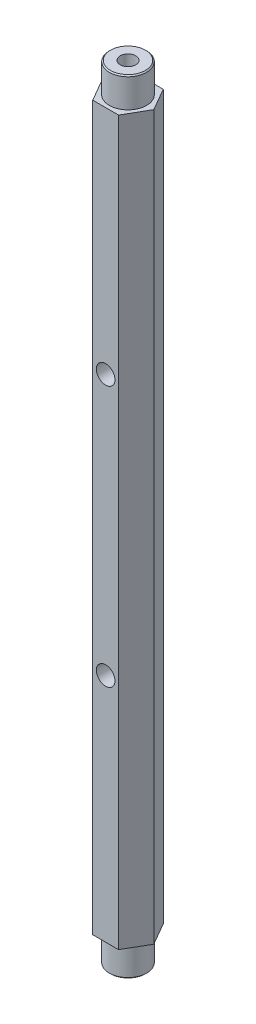
from build123d import *

# Parameters (mm, degrees)
BOSS_EXTRUDE1_DEPTH   = 210
SKETCH2_OUTSIDE_W     = 58.016
SKETCH2_OUTSIDE_H     = 56.16
SKETCH2_OUTSIDE_R     = 5
CUT_EXTRUDE1_DEPTH    = 8
SKETCH3_OUTSIDE_W     = 58.016
SKETCH3_OUTSIDE_H     = 56.16
SKETCH3_OUTSIDE_R     = 5
CUT_EXTRUDE2_DEPTH    = 8
M6_TAPPED_HOLE1_D     = 5
M5_TAPPED_HOLE1_D     = 4.2
M5_TAPPED_HOLE1_DEPTH = 12.4
M5_TAPPED_HOLE1_TIP   = 1.2618073
M5_TAPPED_HOLE2_D     = 4.2
M5_TAPPED_HOLE2_DEPTH = 12.4
M5_TAPPED_HOLE2_TIP   = 1.2618073
CHAMFER1_SIZE         = 0.3


with BuildPart() as part:
    # Sketch1 → Boss-Extrude1 (new body)
    with BuildSketch(Plane(origin=(0, 0, 0), x_dir=(1, 0, 0), z_dir=(0, 1, 0))):
        Polygon((6.92820323, 0), (3.464101615, 6), (-3.464101615, 6), (-6.92820323, 0), (-3.464101615, -6), (3.464101615, -6), align=None)
    extrude(amount=BOSS_EXTRUDE1_DEPTH)

    # Sketch2 outside → Cut-Extrude1 (cut)
    with BuildSketch(Plane(origin=(0, 210, 0), x_dir=(1, 0, 0), z_dir=(0, 1, 0))):
        Rectangle(SKETCH2_OUTSIDE_W, SKETCH2_OUTSIDE_H)
        with Locations(Location((0, 0, 0), (0, 0, 270))):
            Circle(SKETCH2_OUTSIDE_R, mode=Mode.SUBTRACT)
    extrude(amount=-CUT_EXTRUDE1_DEPTH, mode=Mode.SUBTRACT)

    # Sketch3 outside → Cut-Extrude2 (cut)
    with BuildSketch(Plane.XZ):
        Rectangle(SKETCH3_OUTSIDE_W, SKETCH3_OUTSIDE_H)
        with Locations(Location((0, 0, 0), (0, 0, 90))):
            Circle(SKETCH3_OUTSIDE_R, mode=Mode.SUBTRACT)
    extrude(amount=-CUT_EXTRUDE2_DEPTH, mode=Mode.SUBTRACT)

    # M6 Tapped Hole1 (through all)
    with Locations(Plane(origin=(0, 0, -6), x_dir=(-1, 0, 0), z_dir=(0, 0, -1))):
        with Locations((0, 140), (0, 70)):
            Hole(M6_TAPPED_HOLE1_D / 2)

    # M5 Tapped Hole1
    with Locations(Plane.XZ):
        with Locations((0, 0)):
            Hole(M5_TAPPED_HOLE1_D / 2, depth=M5_TAPPED_HOLE1_DEPTH)
            with Locations((0, 0, -(M5_TAPPED_HOLE1_DEPTH + M5_TAPPED_HOLE1_TIP / 2))):  # 118° drill point
                Cone(0, M5_TAPPED_HOLE1_D / 2, M5_TAPPED_HOLE1_TIP, mode=Mode.SUBTRACT)

    # M5 Tapped Hole2
    with Locations(Plane(origin=(0, 210, 0), x_dir=(-1, 0, 0), z_dir=(0, 1, 0))):
        with Locations((0, 0)):
            Hole(M5_TAPPED_HOLE2_D / 2, depth=M5_TAPPED_HOLE2_DEPTH)
            with Locations((0, 0, -(M5_TAPPED_HOLE2_DEPTH + M5_TAPPED_HOLE2_TIP / 2))):  # 118° drill point
                Cone(0, M5_TAPPED_HOLE2_D / 2, M5_TAPPED_HOLE2_TIP, mode=Mode.SUBTRACT)

    # Chamfer1
    chamfer1_edges = [part.edges().sort_by_distance(p)[0] for p in [
        (0, 210, -5),
        (0, 0, -5),
    ]]
    chamfer(chamfer1_edges, length=CHAMFER1_SIZE)


solid = part.part
